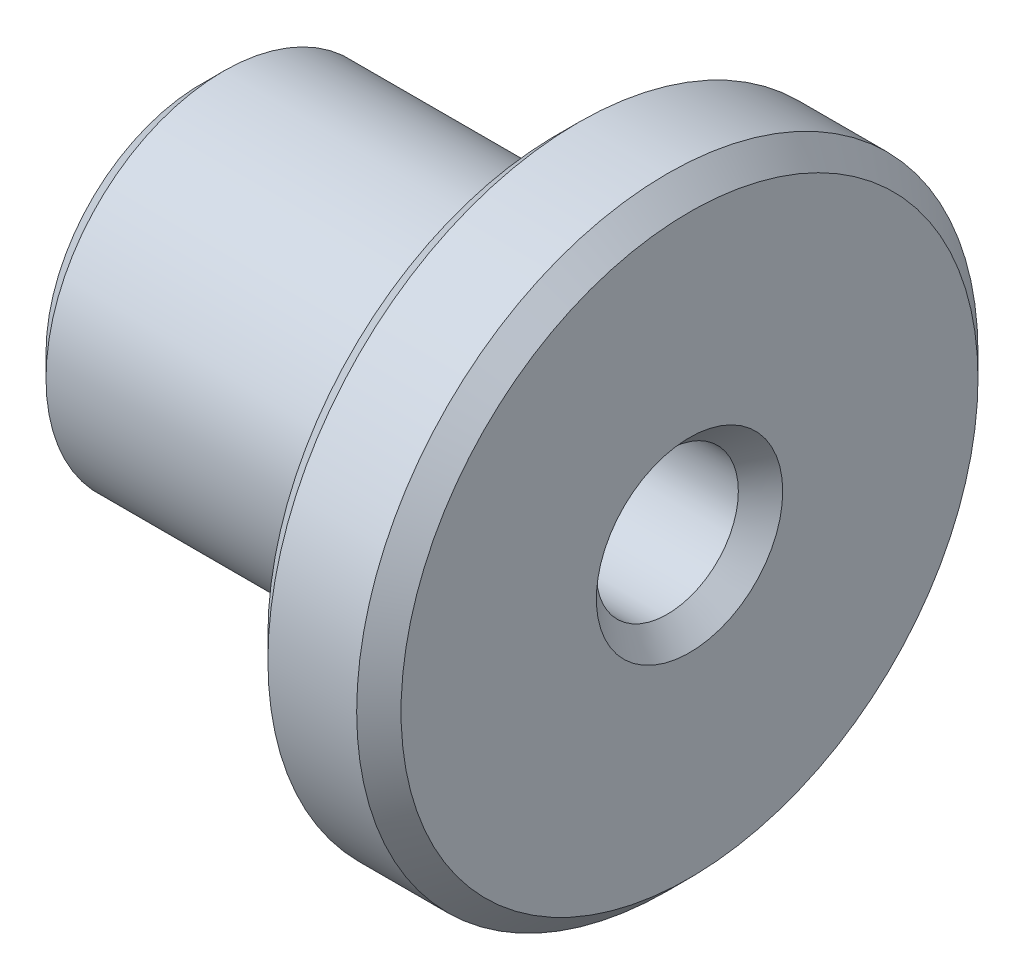
from build123d import *

# Parameters (mm, degrees)
CHAMFER1_SIZE = 0.5


with BuildPart() as part:
    # Sketch1 → Revolve1 (revolve)
    with BuildSketch(Plane.XY, mode=Mode.PRIVATE) as revolve1_sk:
        Polygon((6.5, 30.042572215), (14.5, 30.042572215), (14.5, 33.042572215), (17.5, 33.042572215), (17.5, 27.642572215), (6.5, 27.642572215), align=None)
    revolve(revolve1_sk.sketch.rotate(Axis((17.5, 26.042572215, 0), (-1, 0, 0)), 90), axis=Axis((17.5, 26.042572215, 0), (-1, 0, 0)))

    # Chamfer1
    chamfer1_edges = [part.edges().sort_by_distance(p)[0] for p in [
        (17.5, 26.042572215, 7),
        (14.5, 26.042572215, 7),
        (6.5, 26.042572215, 4),
        (17.5, 26.042572215, 1.6),
    ]]
    chamfer(chamfer1_edges, length=CHAMFER1_SIZE)


solid = part.part
